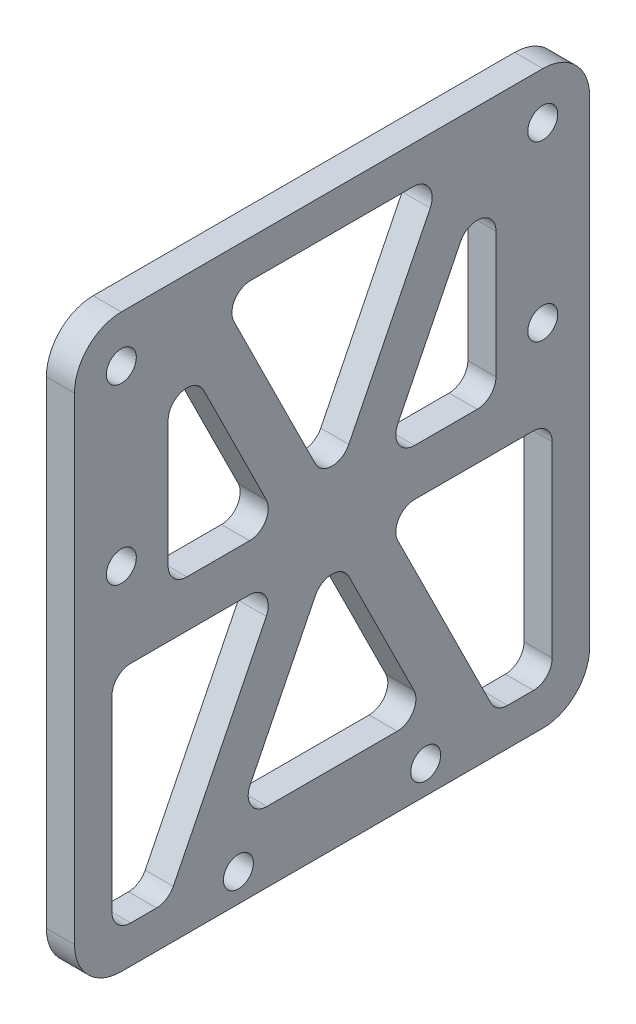
SolidWorks part; units mm, degrees
material "哈碳纤"
ref_plane "前视基准面" through (0, 0, 0) normal (0, 0, 1) x (1, 0, 0)
ref_plane "上视基准面" through (0, 0, 0) normal (0, 1, 0) x (1, 0, 0)
ref_plane "右视基准面" through (0, 0, 0) normal (1, 0, 0) x (0, 0, -1)
other "Configuration Table"
sketch "草图2" plane through (0, 0, 0) normal (1, 0, 0) x (0, 0, -1)
  line L1 (0, 0) -> (55, 0)
  line L2 (0, 0) -> (0, 61)
  line L3 (0, 61) -> (55, 61)
  line L4 (55, 0) -> (55, 61)
  dimension "D1" = 61
  dimension "D2" = 55
extrude "凸台-拉伸1" add sketch "草图2" along normal blind 3
sketch "草图3" plane through (0, 0, 0) normal (-1, 0, 0) x (0, 0, 1)
  line L0 (-55, 61) -> (0, 61) construction
  line L1 (-50, 37.5) -> (-5, 37.5) construction
  line L2 (-50, 37.5) -> (-50, 56) construction
  line L3 (-50, 56) -> (-5, 56) construction
  line L4 (-5, 37.5) -> (-5, 56) construction
  line L6 (-27.5, 61) -> (-27.5, 0) construction
  line L7 (0, 0) -> (-55, 0) construction
  line L9 (-37.5, 3) -> (-17.5, 3) construction
  circle A0 centre (-5, 56) radius 1.6
  circle A1 centre (-5, 37.5) radius 1.6
  circle A2 centre (-50, 56) radius 1.6
  circle A3 centre (-50, 37.5) radius 1.6
  circle A4 centre (-37.5, 3) radius 1.6
  circle A5 centre (-17.5, 3) radius 1.6
  point P14 (-27.5, 56)
  point P19 (-27.5, 3)
  dimension "D3" = 3.2
  dimension "D4" = 3.2
  dimension "D5" = 3.2
  dimension "D6" = 3.2
  dimension "D8" = 3.2
  dimension "D9" = 3.2
  dimension "D1" = 18.5
  dimension "D2" = 45
  dimension "D7" = 5
  dimension "D10" = 20
  dimension "D11" = 3
extrude "切除-拉伸1" cut sketch "草图3" against normal blind 3
fillet "圆角1" radius 5 4 edges at (1.5, 61, 0) (1.5, 61, -55) (1.5, 0, 0) (1.5, 0, -55)
sketch "草图4" plane through (0, 0, 0) normal (-1, 0, 0) x (0, 0, 1)
  line L0 (-39.4175, 57) -> (-27.5, 33)
  line L1 (-15.5825, 57) -> (-27.5, 33)
  line L2 (-39.4175, 57) -> (-15.5825, 57)
  line L3 (-1027.5, 30.5) -> (48972.5, 30.5) construction
  line L4 (-27.5, 4.432) -> (-27.5, 49000) construction
  line L5 (-5, 0) -> (-50, 0) construction
  line L6 (-45, 57) -> (-45, 33)
  line L7 (-45, 33) -> (-33.0825, 33)
  line L8 (-33.0825, 33) -> (-45, 57)
  line L9 (-21.9175, 33) -> (-10, 57)
  line L10 (-10, 33) -> (-21.9175, 33)
  line L11 (-10, 57) -> (-10, 33)
  line L12 (972.5, 30.5) -> (-49027.5, 30.5) construction
  line L13 (-50, 61) -> (-5, 61) construction
  line L14 (0, 56) -> (0, 5) construction
  line L15 (-10, 28) -> (-21.9175, 28)
  line L17 (-21.9175, 28) -> (-10, 4)
  line L18 (-37.6795, 7.5) -> (-27.5, 28)
  line L19 (-17.3205, 7.5) -> (-27.5, 28)
  line L21 (-45, 28) -> (-33.0825, 28)
  line L23 (-33.0825, 28) -> (-45, 4)
  line L24 (-37.6795, 7.5) -> (-17.3205, 7.5)
  line L25 (-45, 28) -> (-51, 28)
  line L26 (-51, 28) -> (-51, 4)
  line L27 (-51, 4) -> (-45, 4)
  line L28 (-10, 28) -> (-4, 28)
  line L29 (-4, 4) -> (-10, 4)
  line L30 (-4, 28) -> (-4, 4)
  line L31 (-55, 5) -> (-55, 56) construction
  point P5 (-27.5, 0)
  point P9 (-27.5, 57)
  dimension "D1" = 24
  dimension "D2" = 5
  dimension "D3" = 2.5
  dimension "D4" = 4
  dimension "D5" = 10
  dimension "D6" = 4
  dimension "D7" = 7.5
extrude "切除-拉伸2" cut sketch "草图4" against normal blind 3
fillet "圆角2" radius 2 20 edges at (1.5, 4, -10) (1.5, 28, -21.9175) (1.5, 28, -4) (1.5, 4, -4) (1.5, 7.5, -37.6795) (1.5, 28, -27.5) (1.5, 7.5, -17.3205) (1.5, 33, -27.5) (1.5, 57, -39.4175) (1.5, 57, -15.5825) (1.5, 33, -45) (1.5, 33, -33.0825) (1.5, 57, -10) (1.5, 33, -10) (1.5, 33, -21.9175) (1.5, 28, -33.0825) (1.5, 4, -45) (1.5, 4, -51) (1.5, 28, -51) (1.5, 57, -45)
